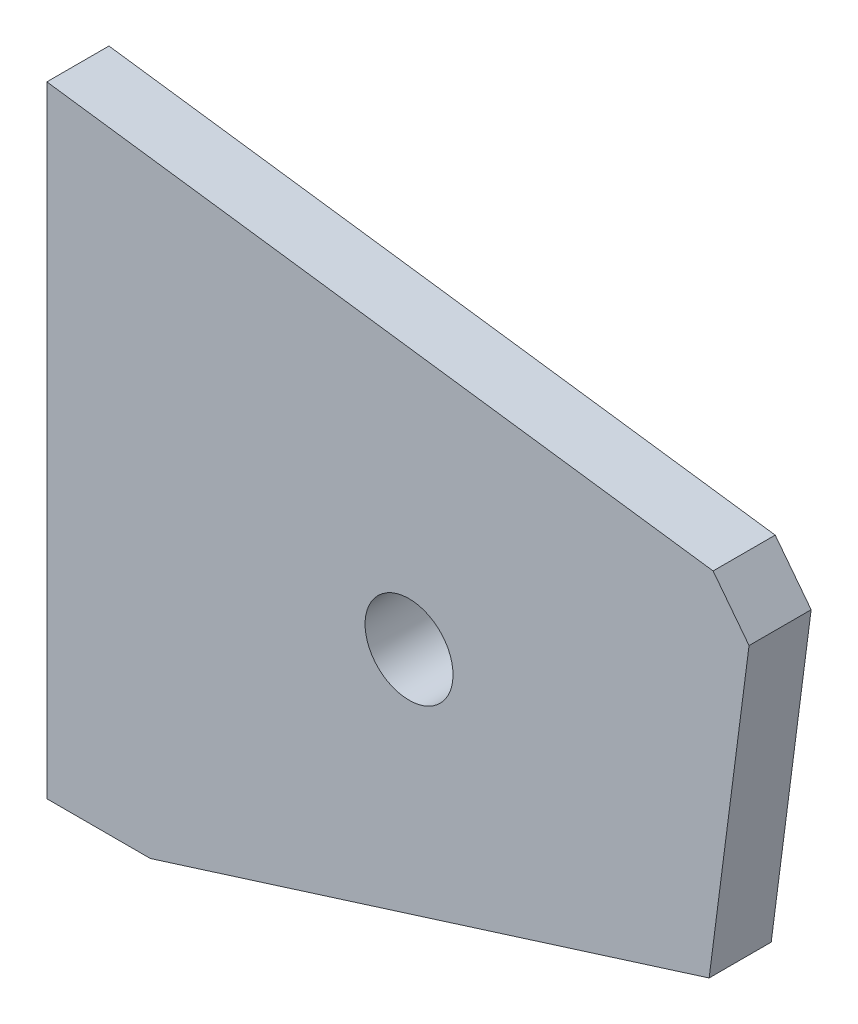
from build123d import *

# Parameters (mm, degrees)
BOSS_EXTRUDE1_DEPTH    = 6
M10_TAPPED_HOLE2_D     = 8.5
M10_TAPPED_HOLE2_DEPTH = 24.5
M10_TAPPED_HOLE2_TIP   = 2.553657631
CHAMFER1_SIZE          = 4
CHAMFER1_SIZE2         = 4.024049749


with BuildPart() as part:
    # Sketch1 → Boss-Extrude1 (new body)
    with BuildSketch(Plane.XY):
        Polygon((0, 0), (0, 60), (68.372865684, 50.718230869), (64, 17), (10, 0), align=None)
    extrude(amount=BOSS_EXTRUDE1_DEPTH)

    # M10 Tapped Hole2
    with Locations(Plane.XY.offset(6)):
        with Locations((35, 30)):
            Hole(M10_TAPPED_HOLE2_D / 2, depth=M10_TAPPED_HOLE2_DEPTH)
            with Locations((0, 0, -(M10_TAPPED_HOLE2_DEPTH + M10_TAPPED_HOLE2_TIP / 2))):  # 118° drill point
                Cone(0, M10_TAPPED_HOLE2_D / 2, M10_TAPPED_HOLE2_TIP, mode=Mode.SUBTRACT)

    # Chamfer1
    chamfer1_edges = [part.edges().sort_by_distance(p)[0] for p in [
        (68.372865684, 50.718230869, 3),
    ]]
    chamfer1_side = [part.faces().sort_by_distance(p)[0] for p in [
        (66.186432842, 33.859115434, 3),
    ]]
    chamfer(chamfer1_edges, length=CHAMFER1_SIZE, length2=CHAMFER1_SIZE2, reference=chamfer1_side[0])


solid = part.part
